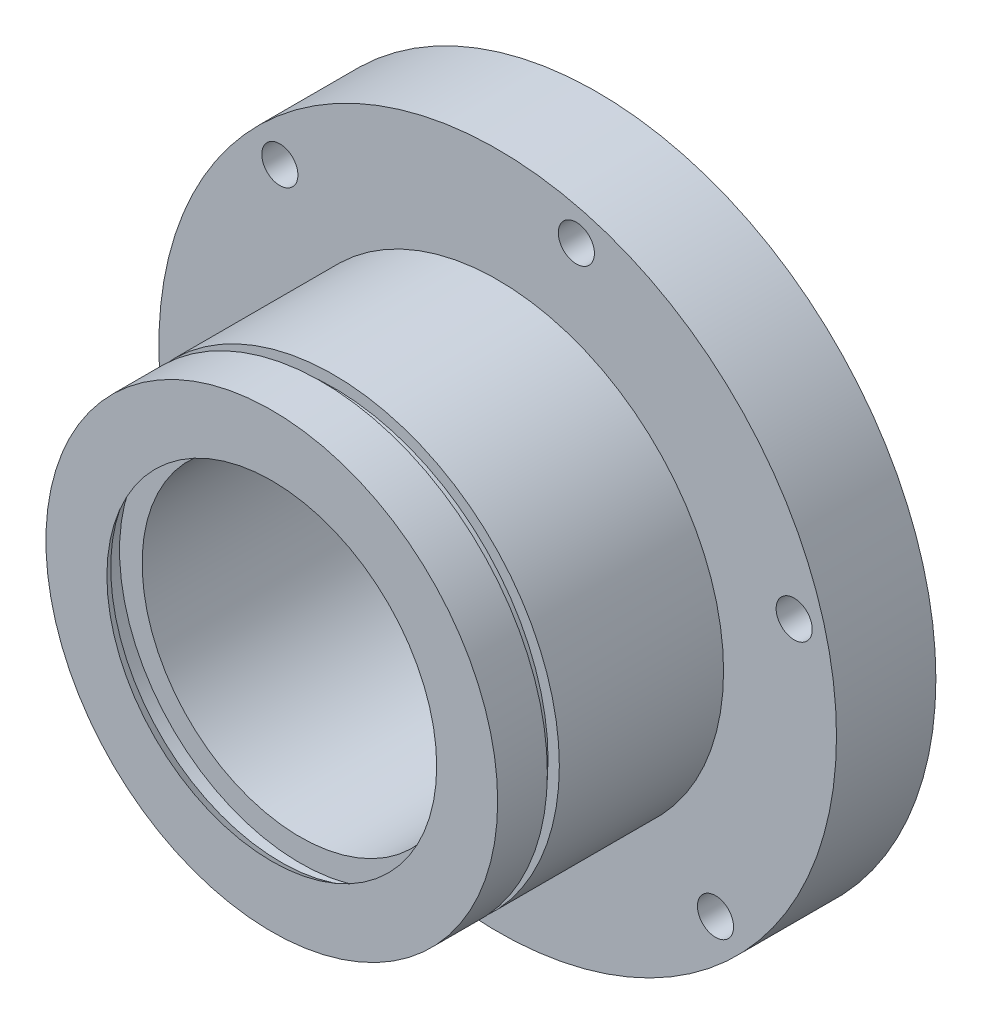
SolidWorks part; units mm, degrees
ref_plane "Front Plane" through (0, 0, 0) normal (0, 0, 1) x (1, 0, 0)
ref_plane "Top Plane" through (0, 0, 0) normal (0, 1, 0) x (1, 0, 0)
ref_plane "Right Plane" through (0, 0, 0) normal (1, 0, 0) x (0, 0, -1)
other "Configuration Table"
sketch "Sketch1" plane through (0, 0, 0) normal (0, 0, 1) x (1, 0, 0)
  circle A0 centre (0, 0) radius 75
  circle A1 centre (0, 0) radius 35
  dimension "D1" = 150
  dimension "D2" = 70
extrude "Boss-Extrude1" add sketch "Sketch1" along normal blind 22
sketch "Sketch2" plane through (0, 0, 0) normal (0, 0, 1) x (1, 0, 0)
  circle A0 centre (0, 0) radius 50
  circle A1 centre (0, 0) radius 35
  dimension "D1" = 100
extrude "Boss-Extrude2" add sketch "Sketch2" along normal blind 50 from offset 22
sketch "Sketch3" plane through (0, 0, 0) normal (0, 0, 1) x (1, 0, 0)
  circle A0 centre (0, 0) radius 50
  circle A1 centre (0, 0) radius 47.5
  dimension "D1" = 95
extrude "Cut-Extrude1" cut sketch "Sketch3" against normal blind 2.65 from offset 61
sketch "Sketch5" plane through (0, 0, 0) normal (0, 0, -1) x (-1, 0, 0)
  circle A0 centre (-17.4139, 65.7324) radius 4
  circle A1 centre (48.219, 47.9471) radius 4
  circle A2 centre (65.6329, -17.7853) radius 4
  circle A3 centre (17.4139, -65.7324) radius 4
  circle A4 centre (-48.219, -47.9471) radius 4
  circle A5 centre (-65.6329, 17.7853) radius 4
  point P16 (0, 0)
  dimension "D2" = 8
  dimension "D1" = 68
  dimension "D3" = 6
extrude "Cut-Extrude2" cut sketch "Sketch5" against normal through all
cosmetic thread "Cosmetic Thread1" parameters "D2"=9
cosmetic thread "Cosmetic Thread2" parameters "D2"=9
cosmetic thread "Cosmetic Thread3" parameters "D2"=9
cosmetic thread "Cosmetic Thread4" parameters "D2"=9
cosmetic thread "Cosmetic Thread5" parameters "D2"=9
cosmetic thread "Cosmetic Thread6" parameters "D2"=9
chamfer "Chamfer1" distance 1 angle 45 6 edges at (44.219, -47.9471, 0) (-21.4139, -65.7324, 0) (-69.6329, -17.7853, 0) (-52.219, 47.9471, 0) (61.6329, 17.7853, 0) (13.4139, 65.7324, 0)
sketch "Sketch7" plane through (0, 0, 0) normal (1, 0, 0) x (0, 0, -1)
  line L0 (-72, 35) -> (-72, 36.5)
  line L1 (-72, 50) -> (-72, -50) construction
  line L3 (-70, 40) -> (-65.7, 40)
  line L4 (-65.7, 40) -> (-65.7, 35)
  line L5 (0, 35) -> (-72, 35) construction
  line L6 (-65.7, 35) -> (-72, 35)
  line L7 (-70, 40) -> (-70, 37.6547)
  line L8 (-70, 37.6547) -> (-72, 36.5)
  line L9 (-72, 0) -> (-61.3501, 0) construction
  dimension "D1" = 5
  dimension "D2" = 2
  dimension "D3" = 6.3
  dimension "D4" = 30
  dimension "D5" = 1.5
revolve "Cut-Revolve1" cut sketch "Sketch7" angle 360 about L9
